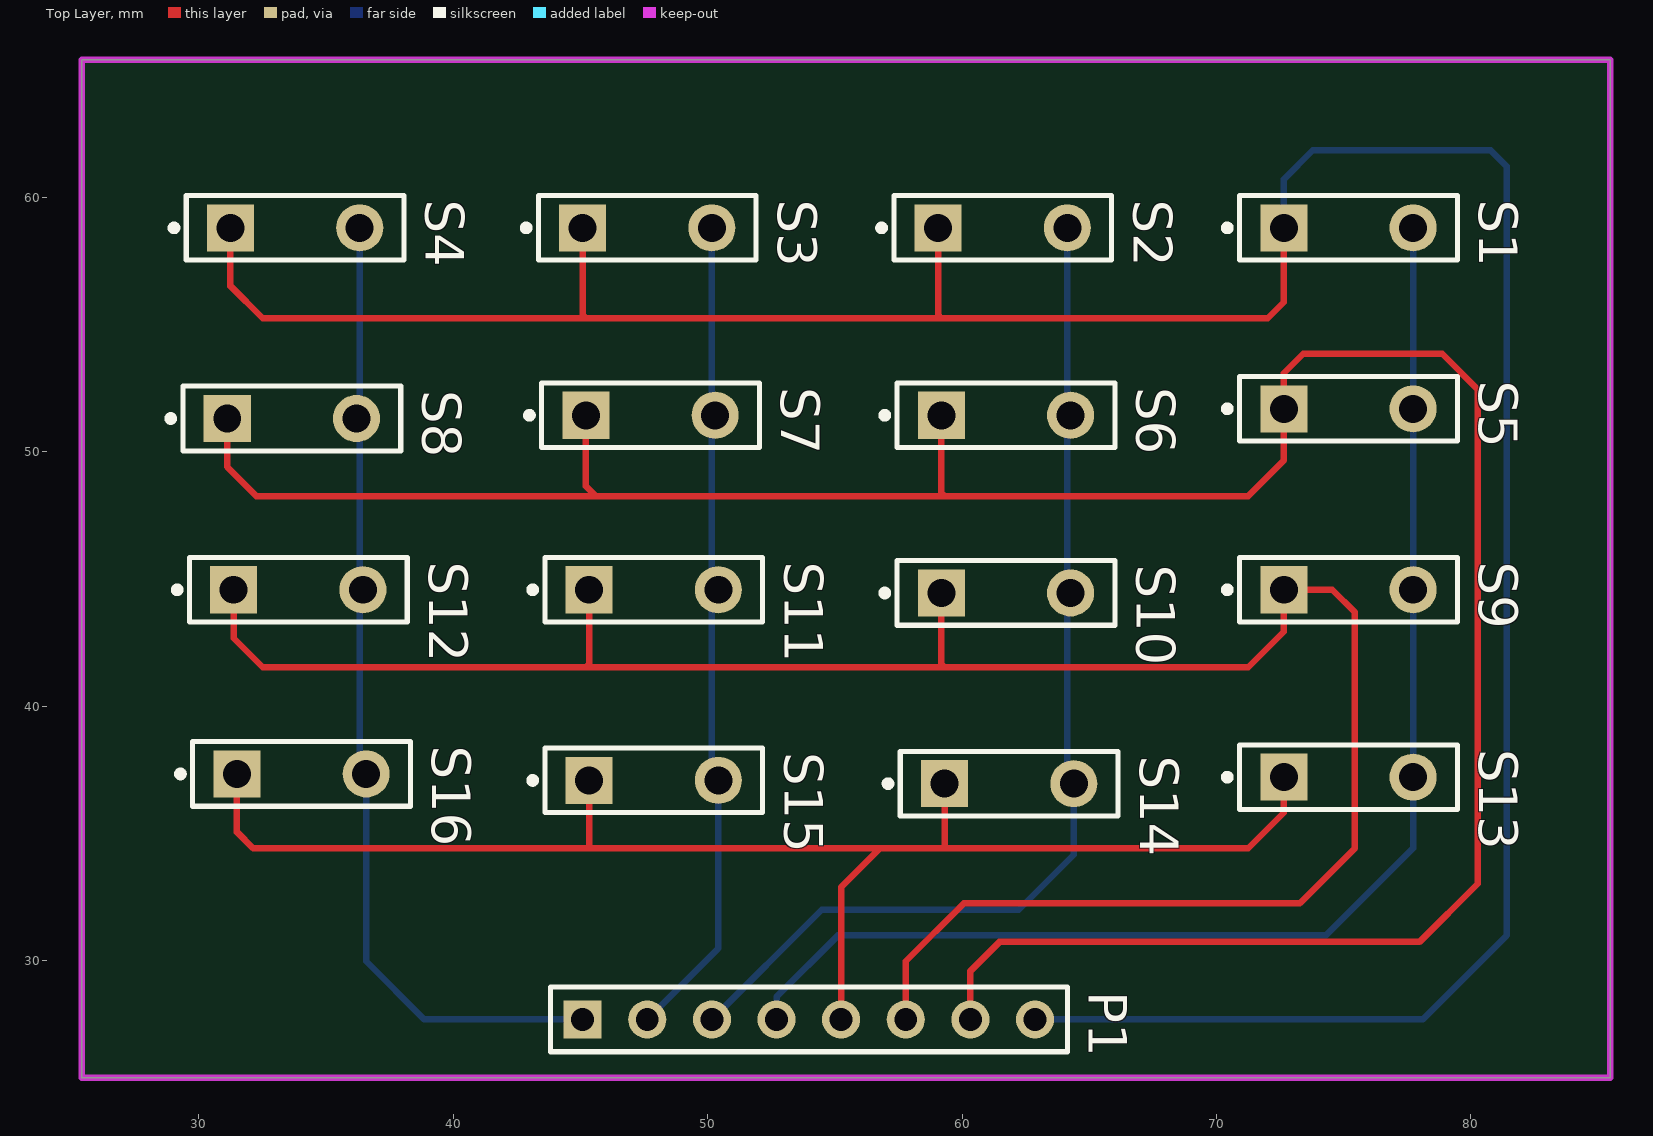
[diagram p0: Top Layer view]
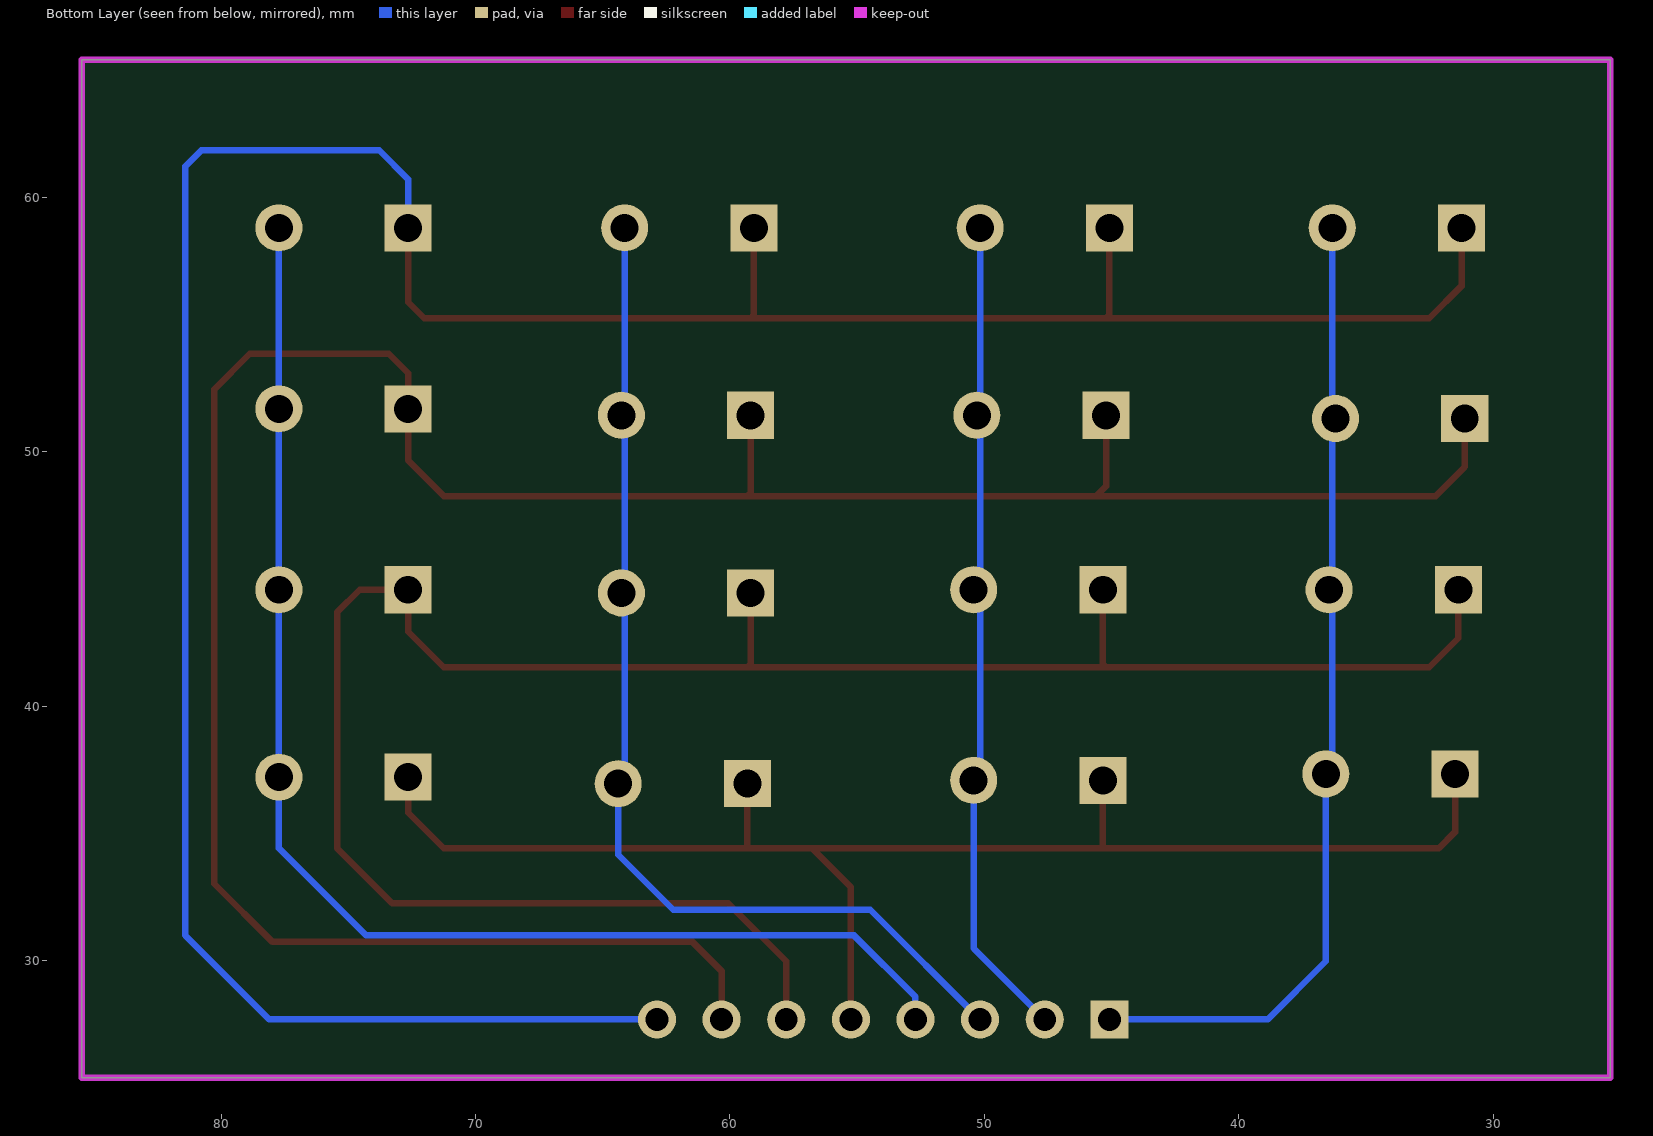
[diagram p1: Bottom Layer view, seen from below]
# Altium PCB MISC80676.PcbDoc
Units mm, origin at the board's own origin, x right, y up, seen from the top; angles counter-clockwise.
Board outline 60.07 x 40 mm, 2 copper layers (Top Layer, Bottom Layer); 17 components, 8 nets, 40 pads, 0 vias.

## Layer stack, top to bottom (the 12.6 mil dielectric is the usual default, probably not edited)
Top Solder: solder mask 0.0102, Solder Resist, Dk 3.5
Top Layer: signal copper 0.0356
Dielectric 1: dielectric 0.32, FR-4, Dk 4.8
Bottom Layer: signal copper 0.0356
Bottom Solder: solder mask 0.0102, Solder Resist, Dk 3.5

## Board outline
25.4,25.4 25.4,65.405 85.471,65.405 85.471,25.4

## Design rules (kind name [scope] priority, off if disabled: settings)
Clearance [All] p1: gap=0.254
MinimumSolderMaskSliver [All] p1: minsoldermaskwidth=0
PolygonConnect [All] p1: connectstyle=Relief reliefconductorwidth=0.254 reliefentries=4 polygonreliefangle="90 Angle" airgapwidth=0.254
RoutingVias [All] p1: holewidth=0.711 width=1.27 viastyle="Through Hole" minholewidth=0.711 minwidth=1.27 maxholewidth=0.711 maxwidth=1.27
SilkToSilkClearance [All] p1: silktosilkclearance=0
SilkToSolderMaskClearance [IsPad] p1: minsilkscreentomaskgap=0 clearancetoexposedcopper=TRUE
SolderMaskExpansion [All] p1: expansion=0.102
Width [All] p1: maxlimit=0.254 minlimit=0.254 preferedwidth=0.254
27 further rules are at their usual default settings.

## Components (designator, comment, footprint, x,y, rotation, side; value= is the part's Value field where it differs from the comment)
P1 "Header 8" HDR1X8 45.085,27.686 r0 top
S1 "SW-PB" SPST-2 75.184,58.801 r0 top
S2 "SW-PB" SPST-2 61.595,58.801 r0 top
S3 "SW-PB" SPST-2 47.625,58.801 r0 top
S4 "SW-PB" SPST-2 33.782,58.801 r0 top
S5 "SW-PB" SPST-2 75.184,51.689 r0 top
S6 "SW-PB" SPST-2 61.722,51.435 r0 top
S7 "SW-PB" SPST-2 47.752,51.435 r0 top
S8 "SW-PB" SPST-2 33.655,51.308 r0 top
S9 "SW-PB" SPST-2 75.184,44.577 r0 top
S10 "SW-PB" SPST-2 61.722,44.45 r0 top
S11 "SW-PB" SPST-2 47.879,44.577 r0 top
S12 "SW-PB" SPST-2 33.909,44.577 r0 top
S13 "SW-PB" SPST-2 75.184,37.211 r0 top
S14 "SW-PB" SPST-2 61.849,36.957 r0 top
S15 "SW-PB" SPST-2 47.879,37.084 r0 top
S16 "SW-PB" SPST-2 34.036,37.338 r0 top

## Footprints (in the part's own frame and the unit in brackets; to place one, negate y for a bottom-side part, rotate by r counter-clockwise, add the part's x,y. Pads: shape width x height; smd on the part's side, far side on the other; paste and mask are expansions set on the pad)
HDR1X8 [mm] "Connector; Header; 8 Position"
  rect 1.5x1.5 hole 0.9: 1(0,0)
  round 1.5 hole 0.9: 2(2.54,0) 3(5.08,0) 4(7.62,0) 5(10.16,0) 6(12.7,0) 7(15.24,0) 8(17.78,0)
  silkscreen extent -1.27,-1.27 19.05,1.27
SPST-2 [mm] "Switch; 2 Leads"
  rect 1.85x1.85 hole 1.1: 1(-2.54,0)
  round 1.85 hole 1.1: 2(2.54,0)
  silkscreen extent -4.89,-1.27 4.28,1.27

## Part data
P1: "Header, 8-Pin"
S1 S2 S3 S4 S5 S6 S7 S8 S9 S10 S11 S12 S13 S14 S15 S16: "Switch"

## Nets (pads, with @x,y where several pads share a name; then routed paths per layer and width w, separated by ;. In a path a pad name is that pad's centre, name@x,y a point inside that pad or via, vN(x,y) a via of type N, cw(c..) or ccw(c..) an arc to the next point about the centre after c; other vN are vias at no path point)
KEY1: P1.8 S1.1 S2.1 S3.1 S4.1 | length 116.2
  Top Layer w0.254: S4.1 31.242,56.515 32.512,55.245 45.212,55.245 ; S3.1 45.085,55.372 45.212,55.245 ; S2.1 59.055,55.372 59.182,55.245 ; S1.1 72.644,55.88 72.009,55.245 59.182,55.245 ; 45.212,55.245 59.182,55.245
  Bottom Layer w0.254: P1.8 78.105,27.686 81.407,30.988 81.407,61.214 80.772,61.849 73.787,61.849 72.644,60.706 S1.1
KEY2: P1.7 S5.1 S6.1 S7.1 S8.1 | length 105.7
  Top Layer w0.254: S8.1 31.115,49.403 32.258,48.26 45.593,48.26 ; S7.1 45.212,48.641 45.593,48.26 ; S6.1 59.182,48.387 59.309,48.26 ; P1.7 60.325,29.591 61.468,30.734 77.978,30.734 80.264,33.02 80.264,52.451 78.867,53.848 73.406,53.848 72.644,53.086 S5.1 72.644,49.657 71.247,48.26 59.309,48.26 ; 45.593,48.26 59.309,48.26
KEY3: P1.6 S9.1 S10.1 S11.1 S12.1 | length 86.2
  Top Layer w0.254: S12.1 31.369,42.672 32.512,41.529 45.212,41.529 ; S11.1 45.339,41.656 45.212,41.529 ; P1.6 57.785,29.972 60.071,32.258 73.279,32.258 75.438,34.417 75.438,43.688 74.549,44.577 S9.1 72.644,42.926 71.247,41.529 59.309,41.529 ; S10.1 59.182,41.656 59.309,41.529 ; 45.212,41.529 59.309,41.529
KEY4: P1.5 S13.1 S14.1 S15.1 S16.1 | length 58.2
  Top Layer w0.254: S16.1 31.496,35.052 32.131,34.417 45.339,34.417 ; S15.1 45.339,34.417 ; P1.5 55.245,32.893 56.769,34.417 ; S14.1 59.309,34.417 ; S13.1 72.644,35.814 71.247,34.417 59.309,34.417 ; 45.339,34.417 56.769,34.417 ; 56.769,34.417 59.309,34.417
KEY5: P1.4 S1.2 S5.2 S9.2 S13.2 | length 52.7
  Bottom Layer w0.254: P1.4 52.705,28.575 55.118,30.988 74.295,30.988 77.724,34.417 S13.2 S9.2 S5.2 S1.2
KEY6: P1.3 S2.2 S6.2 S10.2 S14.2 | length 41.7
  Bottom Layer w0.254: P1.3 54.483,32.004 62.23,32.004 64.389,34.163 S14.2 64.135,37.211 S2.2
KEY7: P1.2 S3.2 S7.2 S11.2 S15.2 | length 32.4
  Bottom Layer w0.254: P1.2 50.419,30.48 S15.2 50.165,37.338 S3.2
KEY8: P1.1 S4.2 S8.2 S12.2 S16.2 | length 38.4
  Bottom Layer w0.254: S4.2 36.322,37.592 S16.2 36.576,29.972 38.862,27.686 P1.1

## Keep-outs
Keep-Out Layer:
  the board outline again, w0.254